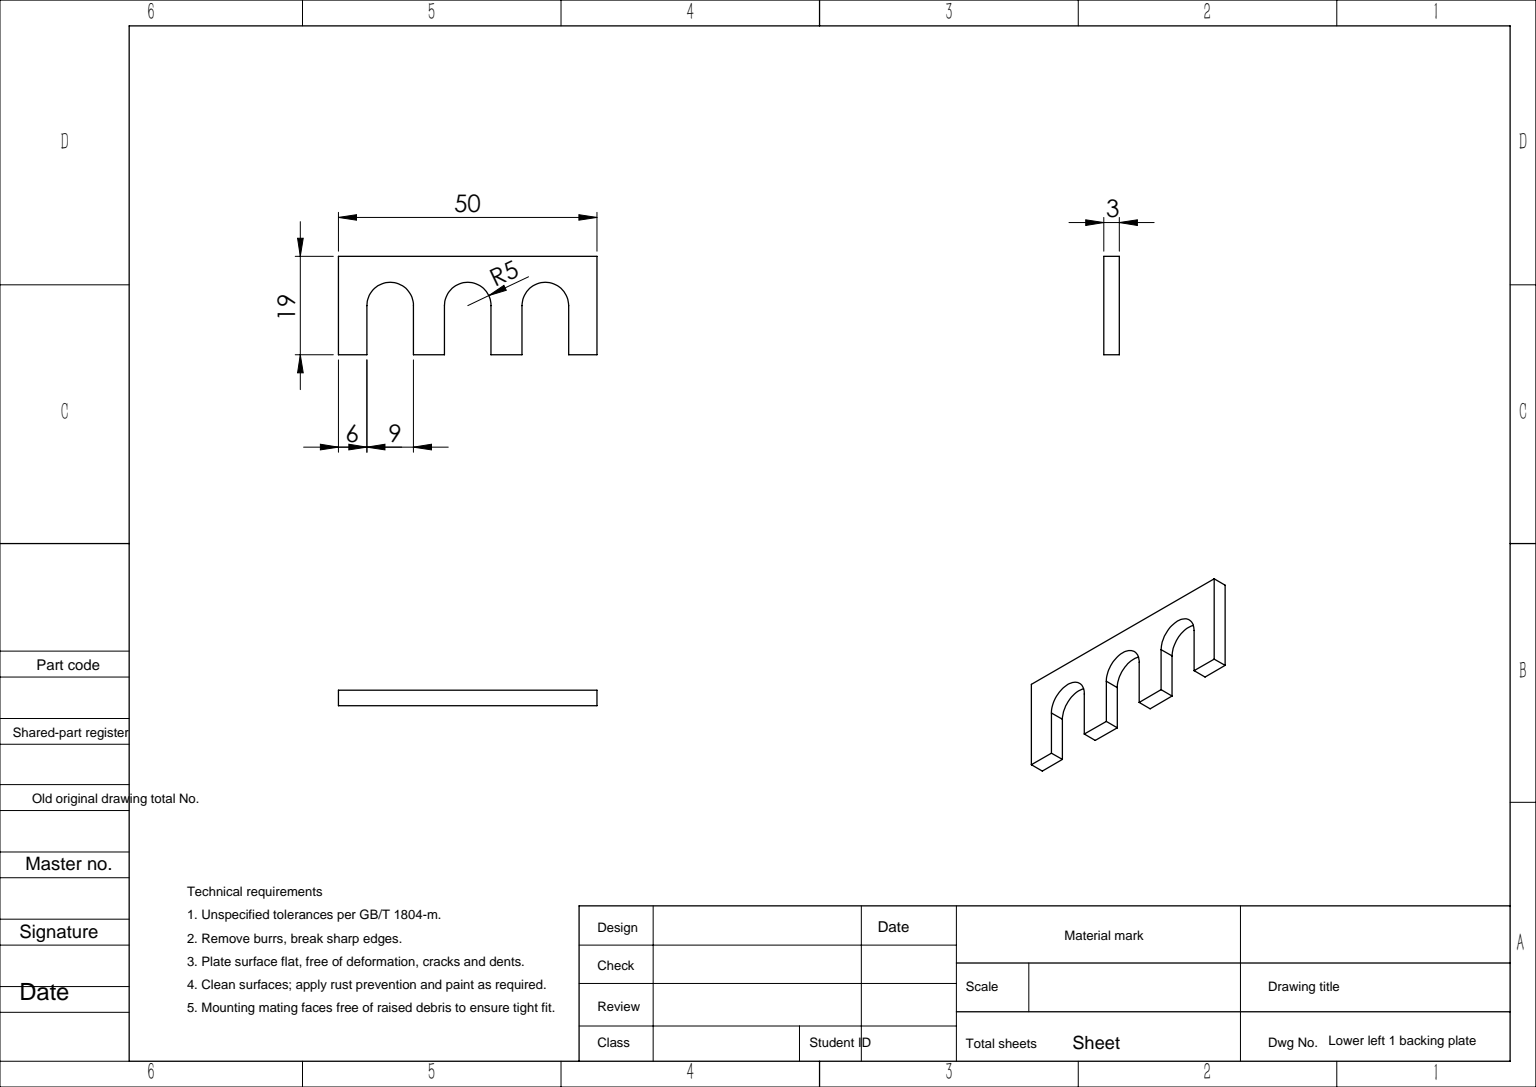
from build123d import *

# Parameters (mm, degrees)
BOSS_EXTRUDE1_DEPTH = 3


with BuildPart() as part:
    # Sketch1 → Boss-Extrude1 (new body)
    with BuildSketch(Plane.XY):
        with BuildLine():
            Line((0, 0), (5.5, 0))
            Line((5.5, 0), (5.5, 9.5))
            ThreePointArc((5.5, 9.5), (10, 14), (14.5, 9.5))
            Line((14.5, 9.5), (14.5, 0))
            Line((14.5, 0), (20.5, 0))
            Line((20.5, 0), (20.5, 9.5))
            ThreePointArc((20.5, 9.5), (25, 14), (29.5, 9.5))
            Line((29.5, 9.5), (29.5, 0))
            Line((29.5, 0), (35.5, 0))
            Line((35.5, 0), (35.5, 9.5))
            ThreePointArc((35.5, 9.5), (40, 14), (44.5, 9.5))
            Line((44.5, 9.5), (44.5, 0))
            Line((44.5, 0), (50, 0))
            Line((50, 0), (50, 19))
            Line((50, 19), (0, 19))
            Line((0, 19), (0, 0))
        make_face()
    extrude(amount=BOSS_EXTRUDE1_DEPTH)


solid = part.part
